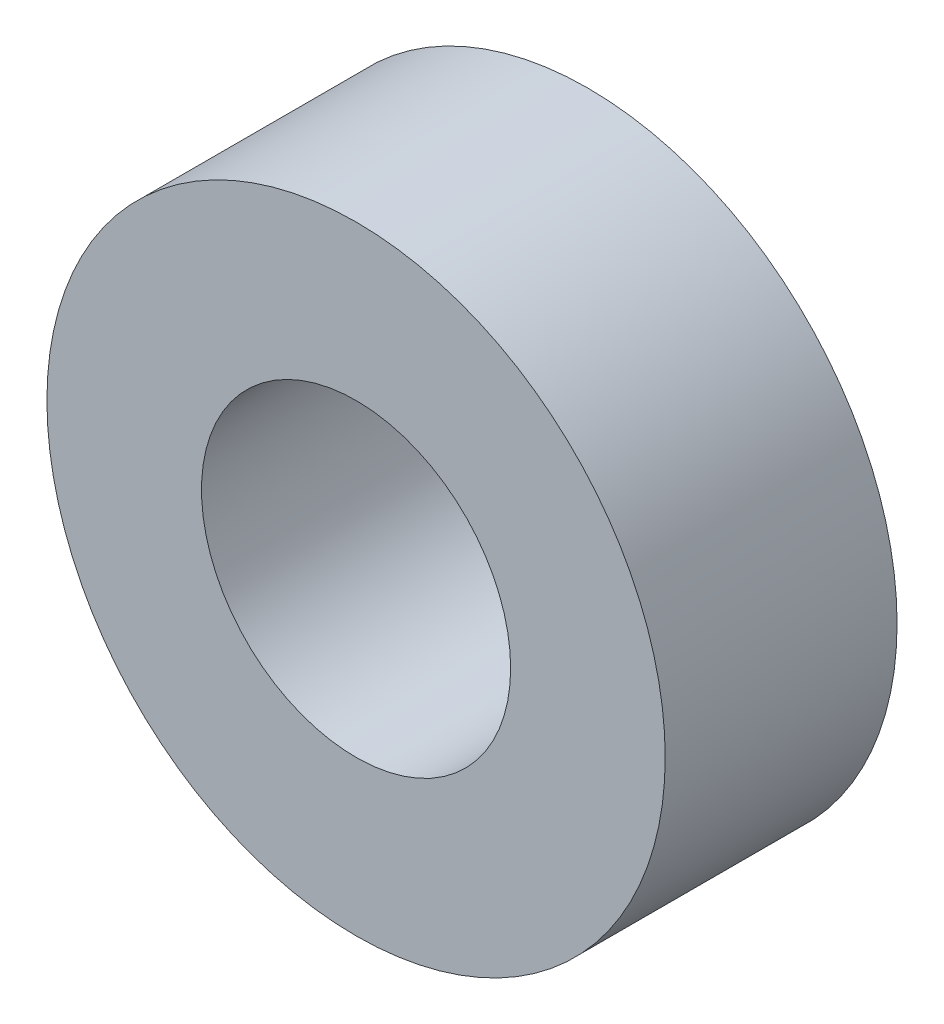
from build123d import *

# Parameters (mm, degrees)
SKETCH_1_R      = 20
SKETCH_1_R_2    = 10
EXTRUDE_1_DEPTH = 7.5


with BuildPart() as part:
    # 草图1 → 凸台-拉伸1 (new, symmetric)
    with BuildSketch(Plane.XY):
        Circle(SKETCH_1_R)
        Circle(SKETCH_1_R_2, mode=Mode.SUBTRACT)
    extrude(amount=EXTRUDE_1_DEPTH, both=True)


solid = part.part
